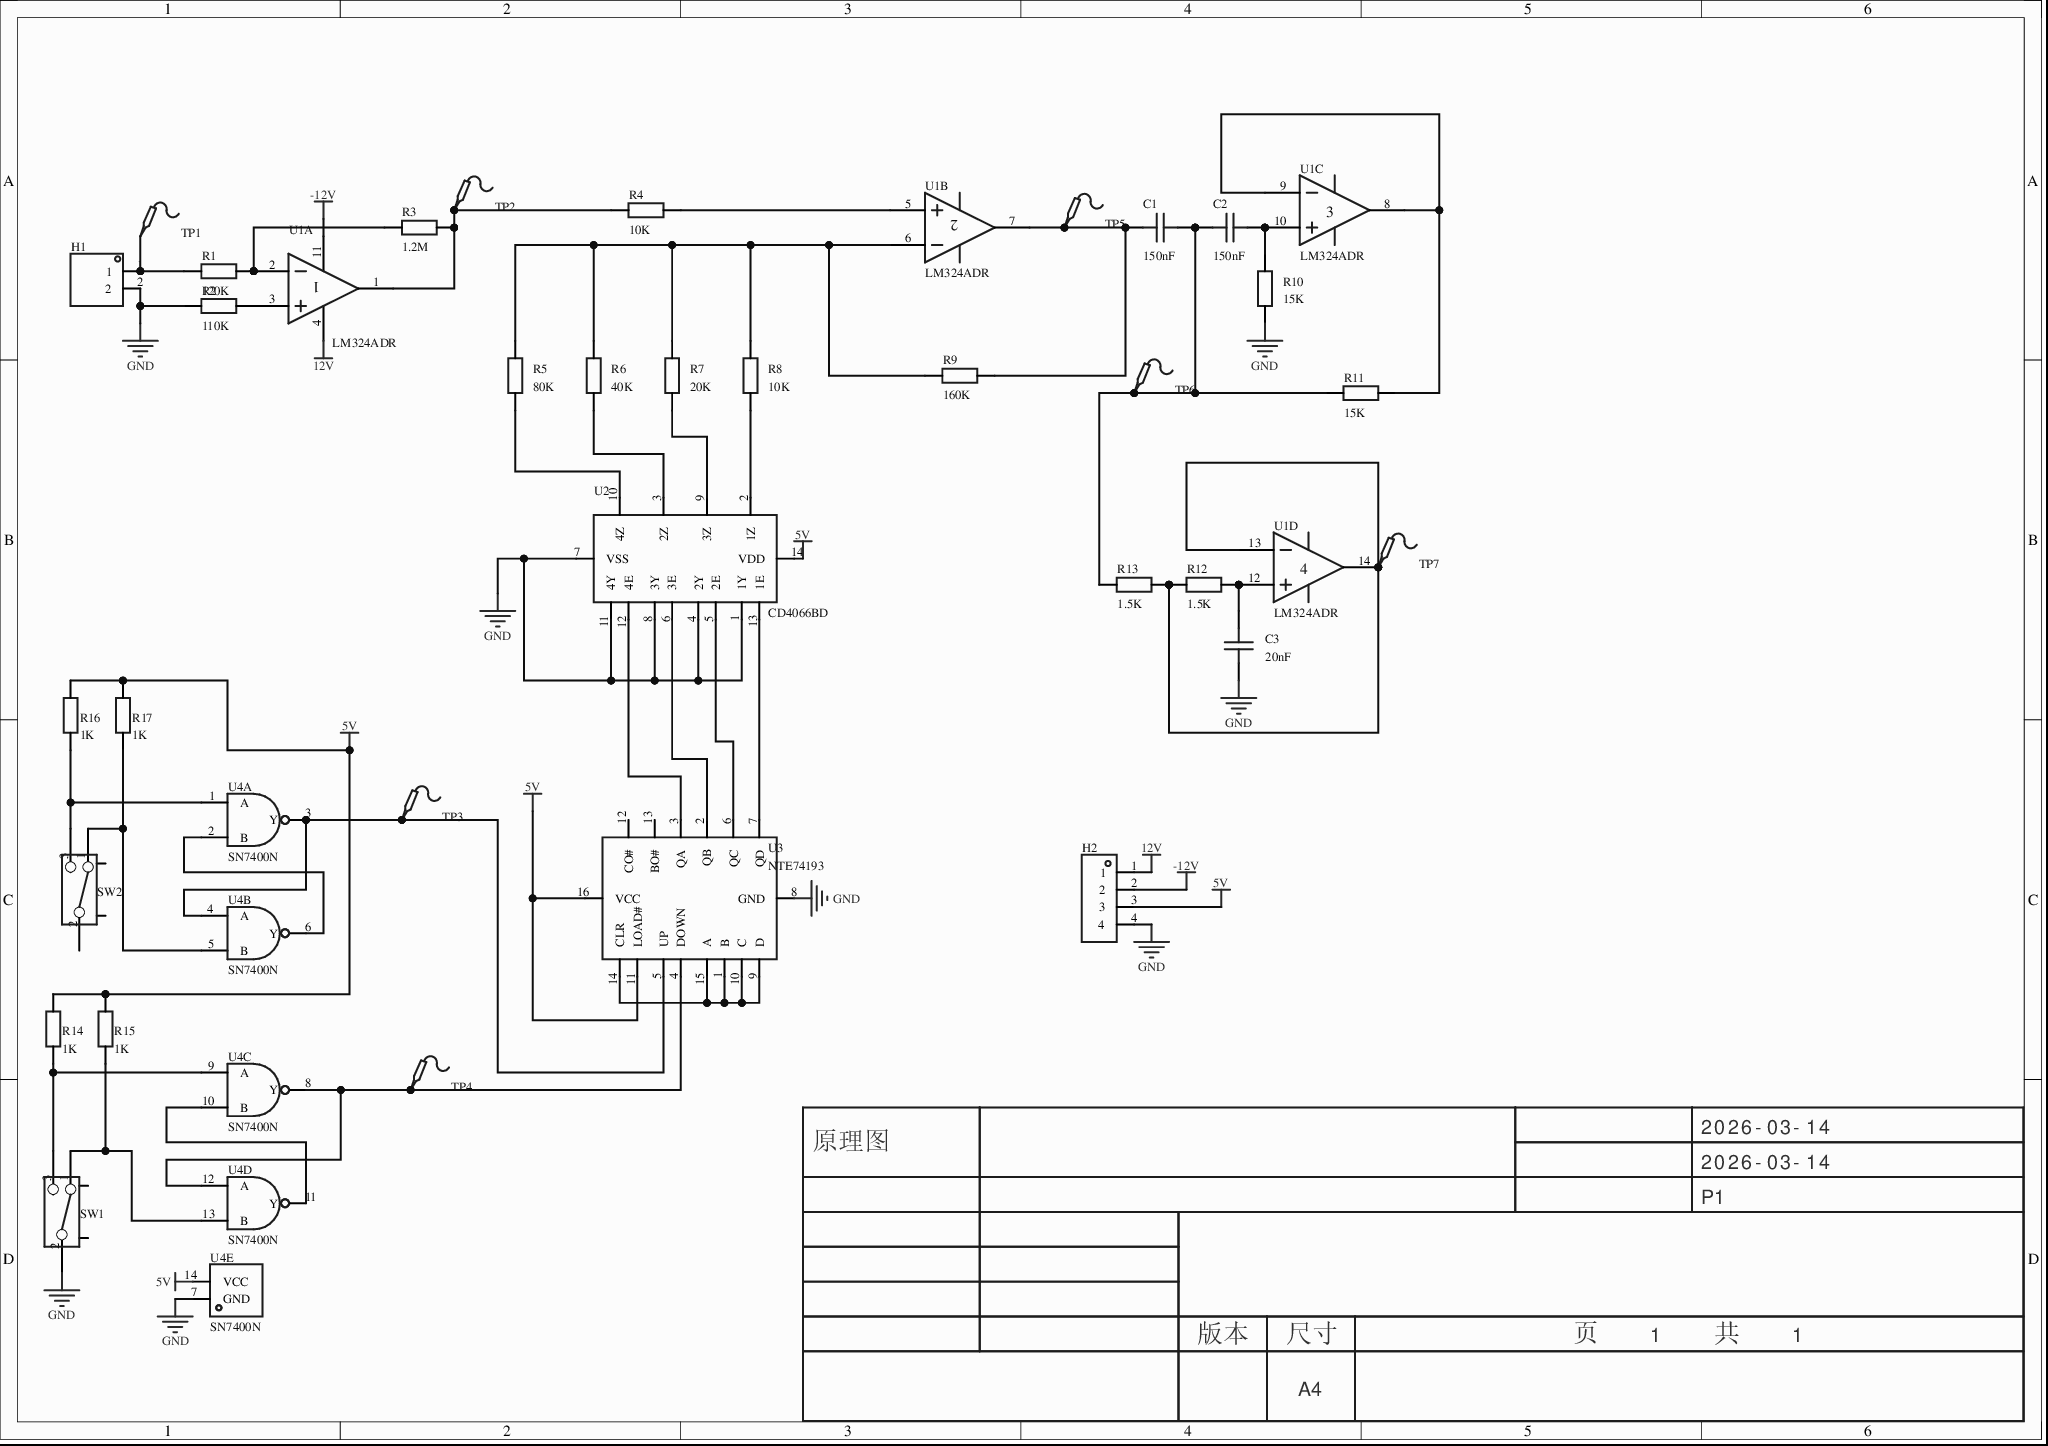
[diagram p0: MISC52011-3.schdoc]
# Altium project MISC52011-2.PrjPcb
1 sheet, 35 parts. Net scope: global (net labels, ports and power ports of the same name join across sheets).
Board file: MISC52011.pcbdoc

## Sheet MISC52011-3.schdoc
size 297 x 209 mm; Version: V1.0; @Project Name: MISC52011; @Update Date: 2026-03-14; @Create Date: 2026-03-14; @Board Name: MISC52011; @Create Time: 16:23:48; @Page Count: 1; @Page No: 1; @Schematic Name: MISC52011; @Update Time: 16:23:48; Size: A4

### Parts
C1  150nF  [C0603]
C2  150nF  [C0603]
C3  20nF  [C0603]
H1  (no value)  [HDR-TH_2P-P2.54-V-M-1]
H2  (no value)  [HDR-TH_4P-P2.54-V-M]
R1  120K  [R0603]
R2  110K  [R0603]
R3  1.2M  [R0603]
R4  10K  [R0603]
R5  80K  [R0603]
R6  40K  [R0603]
R7  20K  [R0603]
R8  10K  [R0603]
R9  160K  [R0603]
R10  15K  [R0603]
R11  15K  [R0603]
R12  1.5K  [R0603]
R13  1.5K  [R0603]
R14  1K  [R0603]
R15  1K  [R0603]
R16  1K  [R0603]
R17  1K  [R0603]
SW1  (no value)  [拨动开关_侧]
SW2  (no value)  [拨动开关_侧]
TP1  (no value)  [Test-Point-0.5mm]
TP2  (no value)  [Test-Point-0.5mm]
TP3  (no value)  [Test-Point-0.5mm]
TP4  (no value)  [Test-Point-0.5mm]
TP5  (no value)  [Test-Point-0.5mm]
TP6  (no value)  [Test-Point-0.5mm]
TP7  (no value)  [Test-Point-0.5mm]
U1  LM324ADR  [SOP-14_L8.6-W3.9-P1.27-LS6.0-BL]  (parts A,B,C,D of 4)
U2  CD4066BD  [SOP-14_L8.6-W3.9-P1.27-LS6.0-BL]
U3  NTE74193  [PDIP-16_L19.7-W6.6-P2.54-LS7.6-BL]
U4  SN7400N  [PDIP-14_L19.3-W6.4-P2.54-LS7.9-BL-1]  (parts A,B,C,D,E of 5)

### Nets
5V: H2.3 R14.2 R15.2 R16.2 R17.2 U2.14(VDD) U3.11(LOAD#) U3.16(VCC) U4.14(VCC)
12V: H2.1 U1.4(VCC)
-12V: H2.2 U1.11(GND)
GND: C3.1 H1.2 H2.4 R2.1 R10.1 SW1.2 U2.1(1Y) U2.4(2Y) U2.7(VSS) U2.8(3Y) U2.11(4Y) U3.8(GND) U4.7(GND)
NetC1_1: C1.1 R9.1 TP5.1 U1.7(2OUT)
NetC1_2: C1.2 C2.1 R11.2 R13.1 TP6.1
NetC2_2: C2.2 R10.2 U1.10(3IN+)
NetC3_2: C3.2 R12.2 U1.12(4IN+)
NetH1_1: H1.1 R1.1 TP1.1
NetR1_2: R1.2 R3.1 U1.2(1IN+)
NetR2_2: R2.2 U1.3(1IN-)
NetR3_2: R3.2 R4.1 TP2.1 U1.1(1OUT)
NetR4_2: R4.2 U1.5(2IN+)
NetR5_1: R5.1 U2.10(4Z)
NetR5_2: R5.2 R6.2 R7.2 R8.2 R9.2 U1.6(2IN-)
NetR6_1: R6.1 U2.3(2Z)
NetR7_1: R7.1 U2.9(3Z)
NetR8_1: R8.1 U2.2(1Z)
NetR11_1: R11.1 U1.8(3OUT) U1.9(3IN-)
NetR12_1: R12.1 R13.2 TP7.1 U1.13(4IN-) U1.14(4OUT)
NetR14_1: R14.1 SW1.3 U4.9(A)
NetR15_1: R15.1 SW1.1 U4.13(B)
NetR16_1: R16.1 SW2.3 U4.1(A)
NetR17_1: R17.1 SW2.1 U4.5(B)
NetTP3_1: TP3.1 U3.5(UP) U4.3(Y) U4.4(A)
NetTP4_1: TP4.1 U3.4(DOWN) U4.8(Y) U4.12(A)
NetU2_5: U2.5(2E) U3.6(QC)
NetU2_6: U2.6(3E) U3.2(QB)
NetU2_12: U2.12(4E) U3.3(QA)
NetU2_13: U2.13(1E) U3.7(QD)
NetU3_1: U3.1(B) U3.9(D) U3.10(C) U3.14(CLR) U3.15(A)
NetU4_2: U4.2(B) U4.6(Y)
NetU4_10: U4.10(B) U4.11(Y)

Not connected (* = marked no-connect by the designer): SW1 4 5; SW2 2 4 5; U3 12(CO#) 13(BO#)

### Notes on the sheet
- 2026-03-14
- 原理图
- P1
- 版本
- 尺寸
- A4
- 页    1    共    1

### Library data of the parts
C1-C3 = CAP_0603: Symbol: Capacitance; ConvertToPcb: yes; ModelId: ac125912035d415993ca9572d50418b10819f05c4eef4c71ace90d822a990e87; ModelName: C0603_L1.6-W0.8-H0.8; ModelTransform: 62.992,31.496,0,0,0,0,0,0,0; Device: CAP_0603; AddInBom: yes; Supplier Footprint: 0603; FootprintName: C0603
  C1 C2: Value: 150nF
  C3: Value: 20nF
H1 = HDR-M_2.54_1x2P: Symbol: 210S-1*2P L=11.6MMGold-plated black; ConvertToPcb: yes; ModelId: 79b2e9f2d70a4d68a1b7098f27c6d4c50819f05c4eef4c71ace90d822a990e87; ModelName: HDR-M-2.54_1x2; ModelTransform: 200,100,0,0,0,0,0,0,-118.11; Device: HDR-M_2.54_1x2P; AddInBom: yes; SupplierPart: C124375; Supplier Footprint: 插件; FootprintName: HDR-TH_2P-P2.54-V-M-1
H2 = HDR-M_2.54_1x4P: Symbol: PZ254V-11-04P; ConvertToPcb: yes; ModelId: 112f4d05e8d64e99ab9a333894bea4f90819f05c4eef4c71ace90d822a990e87; ModelName: HDR-TH_4P-P2.54-M-LI-1X4P; ModelTransform: 399.999,104.7242,0,0,0,0,0,0,-118.11; Device: HDR-M_2.54_1x4P; AddInBom: yes; SupplierPart: C492403; Supplier Footprint: 插件; FootprintName: HDR-TH_4P-P2.54-V-M
R1-R17 = Res_0603: Symbol: 电阻; ConvertToPcb: yes; ModelId: fc143cca1e79419f9cd78b61e9279f080819f05c4eef4c71ace90d822a990e87; ModelTransform: 31.8897,63.7794,0,90,0,0,0,0,0; Device: Res_0603; AddInBom: yes; Supplier Footprint: 0603; FootprintName: R0603; ModelName: R0603
  R1: Value: 120K
  R2: Value: 110K
  R3: Value: 1.2M
  R4 R8: Value: 10K
  R5: Value: 80K
  R6: Value: 40K
  R7: Value: 20K
  R9: Value: 160K
  R10 R11: Value: 15K
  R12 R13: Value: 1.5K
  R14-R17: Value: 1K
SW1 SW2 = 拨动开关_侧: Symbol: 拨动开关; ConvertToPcb: yes; ModelId: 10ea2cc5ba004a75b38812aadef1031f0819f05c4eef4c71ace90d822a990e87; ModelName: SW-TH_SK-12D07-VG3; ModelTransform: 337.98,287.46,295.24,0,0,0,0,-57,-110; Device: 拨动开关_侧; AddInBom: yes; Supplier Footprint: 插件; FootprintName: 拨动开关_侧
TP1-TP7 = Test-Point: Test Point 测试点; AddInBom: yes; Symbol: Test-Point; Device: Test-Point; ConvertToPcb: yes; FootprintName: Test-Point-0.5mm
U1 = LM324ADR_C2837469: 放大器数:四路;轨到轨:-;增益带宽积(GBP):-;输入失调电压(Vos):9mV;输入偏置电流(Ib):250nA;; Manufacturer: UMW(友台半导体); Relevance: []; AddInBom: yes; ModelId: 520b569c4a2341089bdfdd9bf52b86190819f05c4eef4c71ace90d822a990e87; ModelTransform: 339.763,236.22,0,0,0,0,0,0,0; Number of Channels: 四路; Vos - Input Offset Voltage: 9mV; Input Offset Voltage Drift(Vos TC): 7uV/℃; Ib - Input Bias Current: 250nA; Common Mode Rejection Ratio(CMRR): 80dB; Symbol: LM324ADR_C2837469; Device: LM324ADR_C2837469; LCSC Part Name: LM324ADR; SupplierPart: C2837469; ManufacturerPart: LM324ADR; Supplier Footprint: SOP-14; JLCPCB Part Class: Extended Part; Datasheet: https://item.szlcsc.com/datasheet/LM324ADR/3008835.html; Supplier: LCSC; ConvertToPcb: yes; FootprintName: SOP-14_L8.6-W3.9-P1.27-LS6.0-BL; ModelName: SOP-14_L8.6-W3.9-P1.27-LS6.0-BL; Rail to Rail: -; Gain Bandwidth Product: -; Input Offset Current(Ios): -; Input offset current drift(Ios TC): -; Quiescent Current: -; Output Current: -; Operating Temperature: -40℃~+85℃
U2 = CD4066BD: 开关电路:-;导通电阻(Ron):1.05kΩ;; Manufacturer: HTC; AddInBom: yes; ModelId: 520b569c4a2341089bdfdd9bf52b86190819f05c4eef4c71ace90d822a990e87; ModelTransform: 339.763,236.22,0,0,0,0,0,0,0; Voltage - Supply: 3V~18V; Ron: 1.05kΩ; Con: 7.5pF; Bandwidth: 40MHz; Propagation Delay (tpd): 40ns; Symbol: CD4066BD; Device: CD4066BD; LCSC Part Name: CD4066BD; SupplierPart: C558790; ManufacturerPart: CD4066BD; Supplier Footprint: SOP-14; JLCPCB Part Class: Extended Part; Datasheet: https://item.szlcsc.com/datasheet/CD4066BD/582253.html; Supplier: LCSC; ConvertToPcb: yes; FootprintName: SOP-14_L8.6-W3.9-P1.27-LS6.0-BL; ModelName: SOP-14_L8.6-W3.9-P1.27-LS6.0-BL; Switch Circuit: -; Operating Temperature: -55℃~+125℃
U3 = NTE74193: 工作电压:-;元件数:1;计数速率:32MHz;; Manufacturer: NTE ELECTRONICS, INC.; AddInBom: yes; ModelId: 60304d8eb9b246fdb135cb3d16f241a80819f05c4eef4c71ace90d822a990e87; ModelName: PDIP-16_L19.7-W6.6-H5.1-P2.54-LS7.6-BL; ModelTransform: 787.4,311.8104,0,0,0,0,0,0,-118.11; Logic Type: 2分频; Direction: 向下计数器；向上计数器; Number of Elements: 1; Reset: 异步; Timing: 同步; Count Rate: 32MHz; Symbol: NTE74193; Device: NTE74193; LCSC Part Name: NTE74193; SupplierPart: C6345915; ManufacturerPart: NTE74193; Supplier Footprint: PDIP-16; JLCPCB Part Class: Extended Part; Datasheet: https://atta.szlcsc.com/upload/public/pdf/source/20240116/CF6500B458CC39AD140C0B858B31AFAA.pdf; Supplier: LCSC; ConvertToPcb: yes; FootprintName: PDIP-16_L19.7-W6.6-P2.54-LS7.6-BL; Voltage - Supply: -; Operating Temperature: 0℃~+70℃
U4 = SN7400N: 逻辑类型:与非门;通道数:4;电源电压:4.75V~5.25V;最大传播延迟:22ns@5V,15pF;; Manufacturer: TI(德州仪器); Relevance: []; AddInBom: yes; ModelId: 850da569defe42bfb44bffbf615858220819f05c4eef4c71ace90d822a990e87; ModelTransform: 751.967,309.842,0,0,0,0,0,0,-118.11; Logic Gate Type: 与非门; Number of Channels: 4; Sink Current: 16mA; Source Current: 400uA; High Level Range (VIH): 2V; Low Level Range (VIL): 800mV; Symbol: SN7400N; Device: SN7400N; LCSC Part Name: SN7400N; SupplierPart: C2860604; ManufacturerPart: SN7400N; Supplier Footprint: PDIP-14; JLCPCB Part Class: Extended Part; Datasheet: https://www.ti.com/cn/lit/gpn/sn74ls00; Supplier: LCSC; ConvertToPcb: yes; FootprintName: PDIP-14_L19.3-W6.4-P2.54-LS7.9-BL-1; ModelName: PDIP-14_L19.3-W6.4-P2.54-LS7.9-BL-1; Supply Voltage: 4.75V~5.25V; Series: 7400系列; Propagation Delay Time: 22ns@5V,15pF; Operating Temperature: 0℃~+70℃